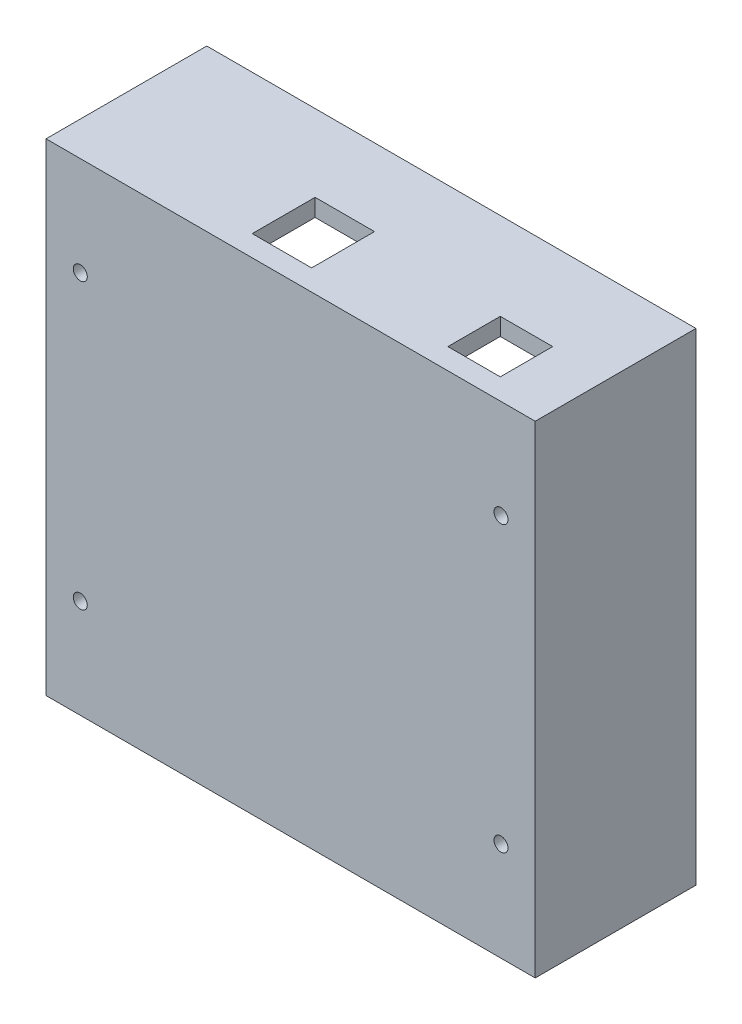
from build123d import *

# Parameters (mm, degrees)
SKETCH1_W           = 140
SKETCH1_H           = 138
BOSS_EXTRUDE1_DEPTH = 46
SHELL1_T            = -5
SKETCH9_W           = 10
SKETCH9_H           = 10
CUT_EXTRUDE2_DEPTH  = 5
SKETCH10_W          = 31
SKETCH10_H          = 22
CUT_EXTRUDE3_DEPTH  = 5
SKETCH11_W          = 17
SKETCH11_H          = 18
CUT_EXTRUDE4_DEPTH  = 5
SKETCH12_W          = 32
SKETCH12_H          = 13
CUT_EXTRUDE5_DEPTH  = 5
SKETCH13_W          = 15
SKETCH13_H          = 15
CUT_EXTRUDE6_DEPTH  = 5
SKETCH19_R          = 2
CUT_EXTRUDE8_DEPTH  = 5
SKETCH21_W          = 16
SKETCH21_H          = 16
CUT_EXTRUDE11_DEPTH = 5
SKETCH23_W          = 16
SKETCH23_H          = 16
CUT_EXTRUDE12_DEPTH = 5
SKETCH24_W          = 10
SKETCH24_H          = 10
SKETCH24_W_2        = 31
SKETCH24_H_2        = 22
SKETCH24_W_3        = 32
SKETCH24_H_3        = 13
BOSS_EXTRUDE2_DEPTH = 5


with BuildPart() as part:
    # Sketch1 → Boss-Extrude1 (new body)
    with BuildSketch(Plane.XY):
        with Locations((22.688228496, 49.11153309)):
            Rectangle(SKETCH1_W, SKETCH1_H)
    extrude(amount=BOSS_EXTRUDE1_DEPTH)

    # Shell1
    shell1_openings = [part.faces().sort_by_distance(p)[0] for p in [
        (22.688228496, 49.11153309, 0),
    ]]
    offset(amount=SHELL1_T, openings=shell1_openings, kind=Kind.INTERSECTION)

    # Sketch9 → Cut-Extrude2 (cut)
    with BuildSketch(Plane(origin=(0, 118.11153309, 0), x_dir=(1, 0, 0), z_dir=(0, 1, 0))):
        with Locations((-34.311771504, -35)):
            Rectangle(SKETCH9_W, SKETCH9_H)
    extrude(amount=-CUT_EXTRUDE2_DEPTH, mode=Mode.SUBTRACT)

    # Sketch10 → Cut-Extrude3 (cut)
    with BuildSketch(Plane(origin=(0, 118.11153309, 0), x_dir=(1, 0, 0), z_dir=(0, 1, 0))):
        with Locations((-11.811771504, -29)):
            Rectangle(SKETCH10_W, SKETCH10_H)
    extrude(amount=-CUT_EXTRUDE3_DEPTH, mode=Mode.SUBTRACT)

    # Sketch11 → Cut-Extrude4 (cut)
    with BuildSketch(Plane(origin=(0, 118.11153309, 0), x_dir=(1, 0, 0), z_dir=(0, 1, 0))):
        with Locations((14.188228496, -31)):
            Rectangle(SKETCH11_W, SKETCH11_H)
    extrude(amount=-CUT_EXTRUDE4_DEPTH, mode=Mode.SUBTRACT)

    # Sketch12 → Cut-Extrude5 (cut)
    with BuildSketch(Plane(origin=(0, 118.11153309, 0), x_dir=(1, 0, 0), z_dir=(0, 1, 0))):
        with Locations((42.688228496, -33.5)):
            Rectangle(SKETCH12_W, SKETCH12_H)
    extrude(amount=-CUT_EXTRUDE5_DEPTH, mode=Mode.SUBTRACT)

    # Sketch13 → Cut-Extrude6 (cut)
    with BuildSketch(Plane(origin=(0, 118.11153309, 0), x_dir=(1, 0, 0), z_dir=(0, 1, 0))):
        with Locations((69.188228496, -32.5)):
            Rectangle(SKETCH13_W, SKETCH13_H)
    extrude(amount=-CUT_EXTRUDE6_DEPTH, mode=Mode.SUBTRACT)

    # Sketch19 → Cut-Extrude8 (cut)
    with BuildSketch(Plane.XY.offset(46)):
        with Locations((-37.511771504, 8.41153309)):
            Circle(SKETCH19_R)
        with Locations((-37.511771504, 89.81153309)):
            Circle(SKETCH19_R)
        with Locations((82.888228496, 8.41153309)):
            Circle(SKETCH19_R)
        with Locations((82.888228496, 89.81153309)):
            Circle(SKETCH19_R)
    extrude(amount=-CUT_EXTRUDE8_DEPTH, mode=Mode.SUBTRACT)

    # Sketch21 → Cut-Extrude11 (cut)
    with BuildSketch(Plane.XZ.offset(19.88846691)):
        with Locations((-20.311771504, 32)):
            Rectangle(SKETCH21_W, SKETCH21_H)
    extrude(amount=-CUT_EXTRUDE11_DEPTH, mode=Mode.SUBTRACT)

    # Sketch23 → Cut-Extrude12 (cut)
    with BuildSketch(Plane.XZ.offset(19.88846691)):
        with Locations((-0.311771504, 32)):
            Rectangle(SKETCH23_W, SKETCH23_H)
    extrude(amount=-CUT_EXTRUDE12_DEPTH, mode=Mode.SUBTRACT)

    # Sketch24 → Boss-Extrude2 (add)
    with BuildSketch(Plane(origin=(0, 118.11153309, 0), x_dir=(1, 0, 0), z_dir=(0, 1, 0))):
        with Locations((-34.311771504, -35)):
            Rectangle(SKETCH24_W, SKETCH24_H)
        with Locations((-11.811771504, -29)):
            Rectangle(SKETCH24_W_2, SKETCH24_H_2)
        with Locations((42.688228496, -33.5)):
            Rectangle(SKETCH24_W_3, SKETCH24_H_3)
    extrude(amount=-BOSS_EXTRUDE2_DEPTH)


solid = part.part
